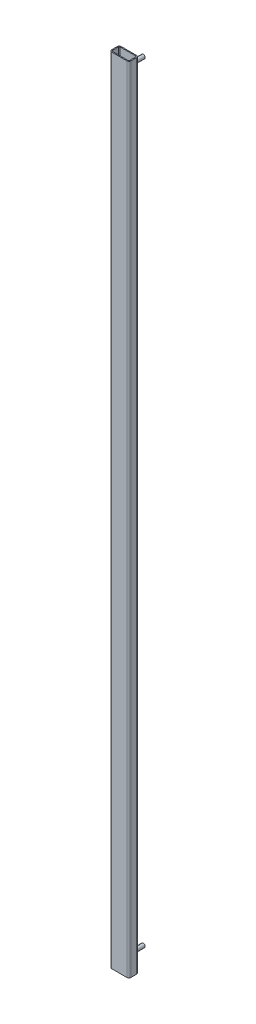
SolidWorks part; units mm, degrees
ref_plane "Front" through (0, 0, 0) normal (0, 0, 1) x (1, 0, 0)
ref_plane "Top" through (0, 0, 0) normal (0, 1, 0) x (1, 0, 0)
ref_plane "Right" through (0, 0, 0) normal (1, 0, 0) x (0, 0, -1)
sketch "草图1" plane through (0, 0, 0) normal (0, 1, 0) x (1, 0, 0)
  line L0 (-16, -8) -> (16, -8)
  line L1 (-16, -10) -> (16, -10)
  line L2 (-20, -6) -> (-20, 6)
  line L3 (-16, 10) -> (16, 10)
  line L4 (20, -6) -> (20, 6)
  line L5 (-20, -10) -> (20, 10) construction
  line L6 (-20, 10) -> (20, -10) construction
  line L7 (18, -6) -> (18, 6)
  line L8 (-16, 8) -> (16, 8)
  line L9 (-18, -6) -> (-18, 6)
  arc A0 (-16, -10) -> (-20, -6) centre (-16, -6) cw
  arc A1 (16, -10) -> (20, -6) centre (16, -6) ccw
  arc A2 (16, 10) -> (20, 6) centre (16, 6) cw
  arc A3 (-20, 6) -> (-16, 10) centre (-16, 6) cw
  arc A4 (16, -8) -> (18, -6) centre (16, -6) ccw
  arc A5 (16, 8) -> (18, 6) centre (16, 6) cw
  arc A6 (-18, 6) -> (-16, 8) centre (-16, 6) cw
  arc A7 (-16, -8) -> (-18, -6) centre (-16, -6) cw
  point P0 (0, 0)
  dimension "D3" = 4
  dimension "D1" = 40
  dimension "D2" = 20
  dimension "D4" = 2
extrude "凸台-拉伸1" add sketch "草图1" along normal blind 1650
sketch "草图2" plane through (0, 0, -10) normal (0, 0, -1) x (-1, 0, 0)
  line L0 (-16, 1650) -> (16, 1650) construction
  line L1 (-16, 0) -> (16, 0) construction
  circle A0 centre (0, 1625) radius 4
  circle A1 centre (0, 25) radius 4
  dimension "D1" = 8
  dimension "D2" = 25
  dimension "D3" = 25
extrude "凸台-拉伸2" add sketch "草图2" along normal blind 30
